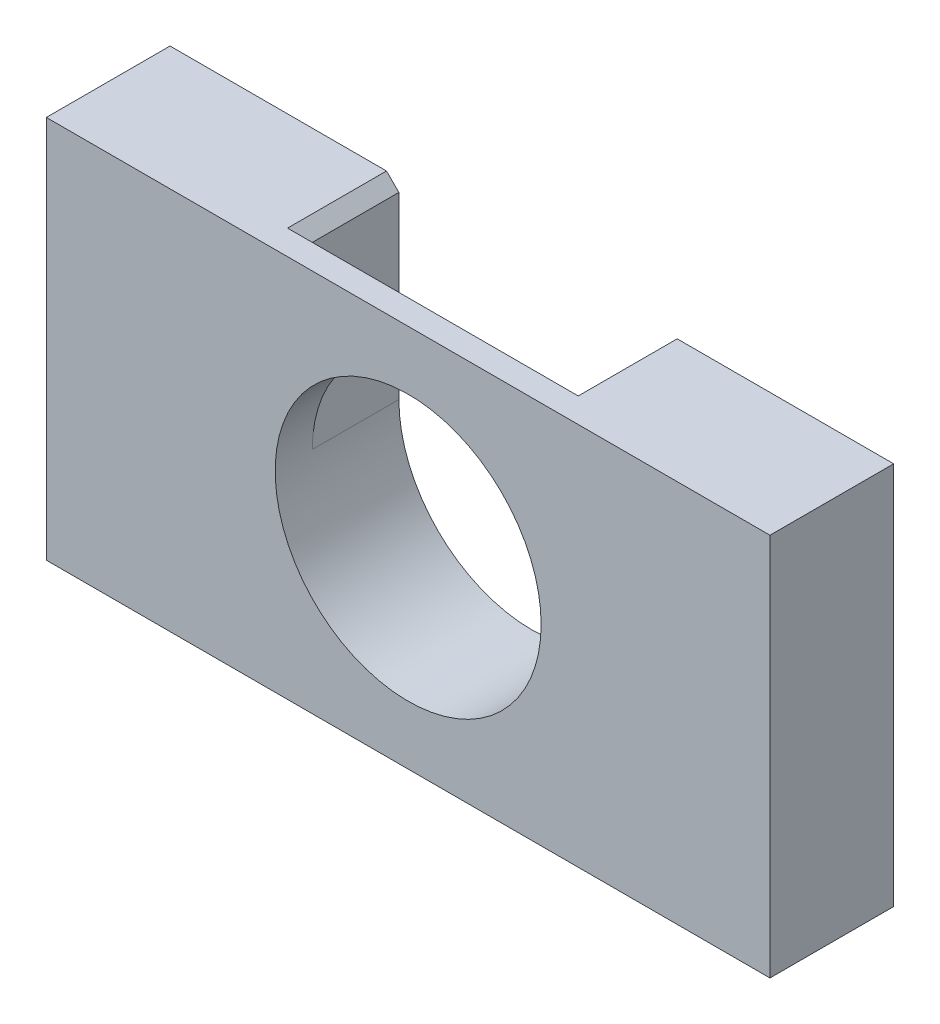
SolidWorks part; units mm, degrees
ref_plane "前视基准面" through (0, 0, 0) normal (0, 0, 1) x (1, 0, 0)
ref_plane "上视基准面" through (0, 0, 0) normal (0, 1, 0) x (1, 0, 0)
ref_plane "右视基准面" through (0, 0, 0) normal (1, 0, 0) x (0, 0, -1)
sketch "草图1" plane through (0, 0, 0) normal (0, 0, 1) x (1, 0, 0)
  line L1 (-58.5, -31) -> (58.5, -31)
  line L2 (-58.5, -31) -> (-58.5, 31)
  line L3 (-58.5, 31) -> (58.5, 31)
  line L4 (58.5, -31) -> (58.5, 31)
  line L5 (-58.5, -31) -> (58.5, 31) construction
  line L6 (-58.5, 31) -> (58.5, -31) construction
  point P0 (0, 0)
  dimension "D1" = 62
  dimension "D2" = 117
extrude "凸台-拉伸1" add sketch "草图1" along normal blind 20
sketch "草图2" plane through (0, 0, 20) normal (0, 0, 1) x (1, 0, 0)
  circle A0 centre (0, 0) radius 21.5
  dimension "D1" = 43
extrude "切除-拉伸1" cut sketch "草图2" against normal up to next
sketch "草图3" plane through (0, 0, 0) normal (0, 0, -1) x (-1, 0, 0)
  line L5 (-58.5, 31) -> (58.5, 31) construction
  line L6 (-21.5, 31) -> (21.5, 31)
  line L7 (-21.5, 31) -> (-21.5, 0)
  line L8 (-21.5, 0) -> (21.5, 0)
  line L9 (21.5, 31) -> (21.5, 0)
  circle A0 centre (0, 0) radius 21.5 construction
  point P5 (0, 0)
  point P7 (21.5, 0)
  point P10 (0, 0)
  point P12 (-21.5, 0)
  point P13 (-21.5, 0)
extrude "切除-拉伸2" cut sketch "草图3" against normal blind 14
chamfer "倒角1" distance 2 angle 45 3 edges at (21.5, 31, 7) (-21.5, 31, 7) (0, 31, 14)
